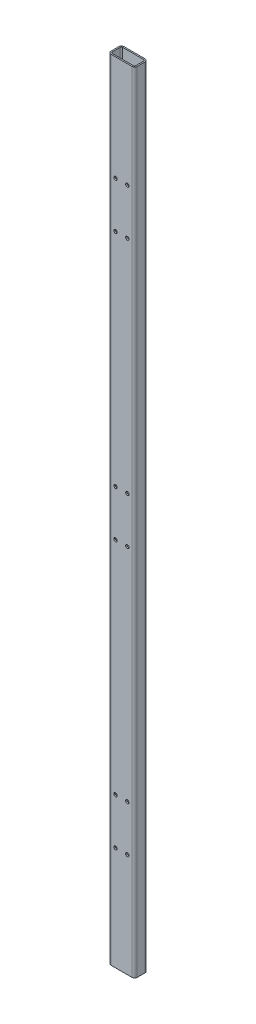
from build123d import *

# Parameters (mm, degrees)
F_40X20X2_1_DEPTH       = 1200
HOLE_WIZARD_5_2_5_2_1_D = 5.2
PATTERN_LINEAR_1_COUNT  = 3
PATTERN_LINEAR_1_PITCH  = 406


with BuildPart() as part:
    # Sketch1 → 矩型管 40X20X2(1) (new body)
    with BuildSketch(Plane.ZX):
        with BuildLine():
            Line((-6, -20), (6, -20))
            ThreePointArc((6, -20), (8.828427125, -18.828427125), (10, -16))
            Line((10, -16), (10, 16))
            ThreePointArc((10, 16), (8.828427125, 18.828427125), (6, 20))
            Line((6, 20), (-6, 20))
            ThreePointArc((-6, 20), (-8.828427125, 18.828427125), (-10, 16))
            Line((-10, 16), (-10, -16))
            ThreePointArc((-10, -16), (-8.828427125, -18.828427125), (-6, -20))
        make_face()
        with BuildLine():
            Line((-6, -18), (6, -18))
            ThreePointArc((6, -18), (7.414213562, -17.414213562), (8, -16))
            Line((8, -16), (8, 16))
            ThreePointArc((8, 16), (7.414213562, 17.414213562), (6, 18))
            Line((6, 18), (-6, 18))
            ThreePointArc((-6, 18), (-7.414213562, 17.414213562), (-8, 16))
            Line((-8, 16), (-8, -16))
            ThreePointArc((-8, -16), (-7.414213562, -17.414213562), (-6, -18))
        make_face(mode=Mode.SUBTRACT)
    extrude(amount=F_40X20X2_1_DEPTH)

    # Ø5.2 (5.2) 直径孔1 (through all)
    with Locations(Plane(origin=(0, 0, -10), x_dir=(-1, 0, 0), z_dir=(0, 0, -1))):
        with Locations((-9, 1040), (9, 1040), (9, 970), (-9, 970)):
            hole_wizard_5_2_5_2_1 = Hole(HOLE_WIZARD_5_2_5_2_1_D / 2)

    # 阵列(线性)1: Ø5.2 (5.2) 直径孔1 ×3
    with Locations(*[(0, -i * PATTERN_LINEAR_1_PITCH, 0) for i in range(1, PATTERN_LINEAR_1_COUNT)]):
        add(hole_wizard_5_2_5_2_1, mode=Mode.SUBTRACT)


solid = part.part
